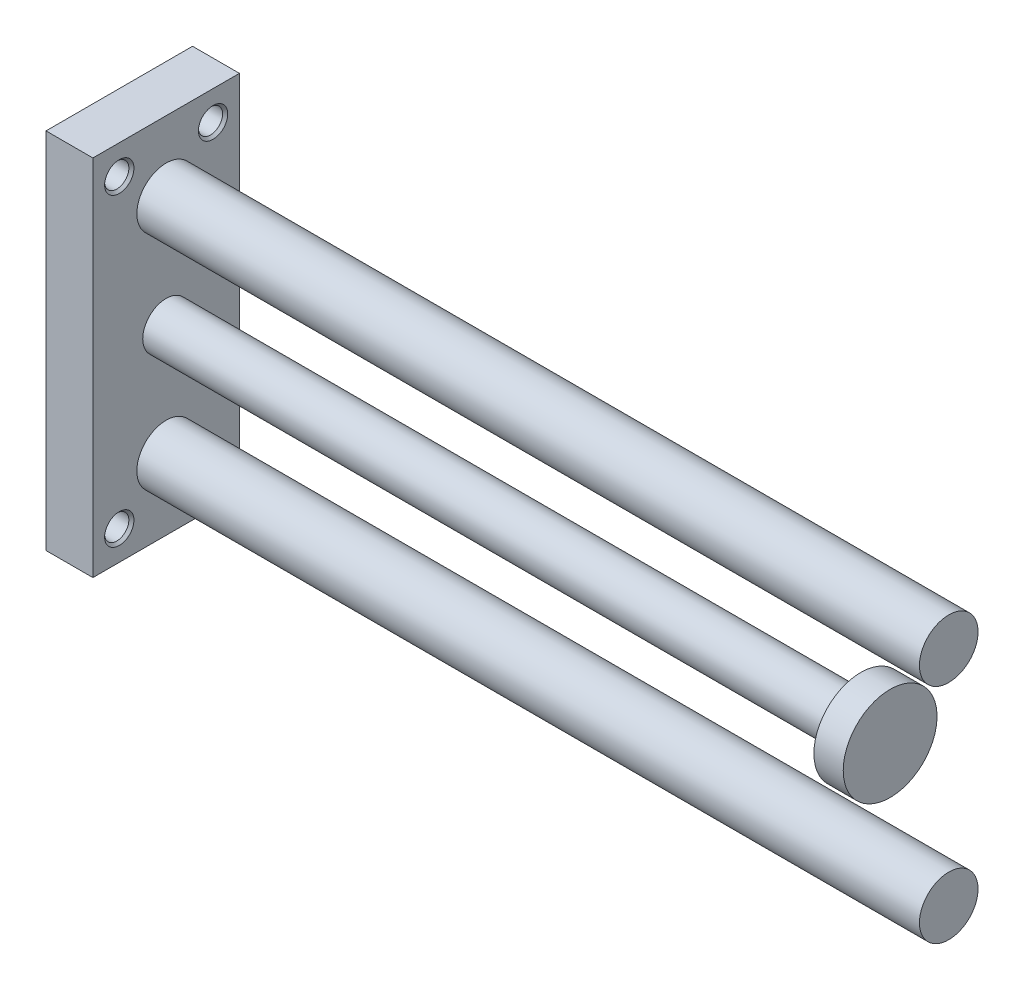
from build123d import *

# Parameters (mm, degrees)
SKETCH_1_W                  = 25
SKETCH_1_H                  = 62
EXTRUDE_1_DEPTH             = 8
SKETCH_2_W                  = 133.5
SKETCH_2_H                  = 5
PATTERN_LINEAR_1_COUNT      = 2
PATTERN_LINEAR_1_PITCH      = 38
PATTERN_LINEAR_2_COUNT      = 2
PATTERN_LINEAR_2_PITCH      = 16
PATTERN_LINEAR_2_COUNT_DIR2 = 2
PATTERN_LINEAR_2_PITCH_DIR2 = 52


with BuildPart() as part:
    # 草图1 → 凸台-拉伸1 (new body)
    with BuildSketch(Plane(origin=(0, 0, 0), x_dir=(0, 0, -1), z_dir=(1, 0, 0))):
        Rectangle(SKETCH_1_W, SKETCH_1_H)
    extrude(amount=-EXTRUDE_1_DEPTH)

    # 草图2 → 旋转1 (revolve)
    with BuildSketch(Plane.XY, mode=Mode.PRIVATE) as revolve_1_sk:
        with Locations((66.75, 21.5)):
            Rectangle(SKETCH_2_W, SKETCH_2_H)
    revolve_1 = revolve(revolve_1_sk.sketch.rotate(Axis((133.5, 19, 0), (-1, 0, 0)), 270), axis=Axis((133.5, 19, 0), (-1, 0, 0)))

    # 阵列(线性)1: 旋转1 ×2
    with Locations(*[(0, -i * PATTERN_LINEAR_1_PITCH, 0) for i in range(1, PATTERN_LINEAR_1_COUNT)]):
        add(revolve_1)

    # 草图4 → 切除-旋转1 (revolve, cut)
    with BuildSketch(Plane.XY.offset(8), mode=Mode.PRIVATE) as cut_revolve_1_sk:
        Polygon((-8, 26), (-8, 28.5), (-7.567, 28.067), (-0.433, 28.067), (0, 28.5), (0, 26), align=None)
    cut_revolve_1 = revolve(cut_revolve_1_sk.sketch.rotate(Axis((0, 26, 8), (-1, 0, 0)), 270), axis=Axis((0, 26, 8), (-1, 0, 0)), mode=Mode.SUBTRACT)

    # 阵列(线性)2: Cut-Revolve 1 2 × 2
    with Locations(*[(0, -j * PATTERN_LINEAR_2_PITCH_DIR2, -i * PATTERN_LINEAR_2_PITCH) for i in range(PATTERN_LINEAR_2_COUNT) for j in range(PATTERN_LINEAR_2_COUNT_DIR2) if (i, j) != (0, 0)]):
        add(cut_revolve_1, mode=Mode.SUBTRACT)

    # 草图6 → 旋转2 (revolve)
    with BuildSketch(Plane.XY, mode=Mode.PRIVATE) as revolve_2_sk:
        Polygon((0, 0), (0, 4), (118.5, 4), (118.5, 8), (123.5, 8), (123.5, 0), align=None)
    revolve(revolve_2_sk.sketch.rotate(Axis((123.5, 0, 0), (-1, 0, 0)), 270), axis=Axis((123.5, 0, 0), (-1, 0, 0)))


solid = part.part
